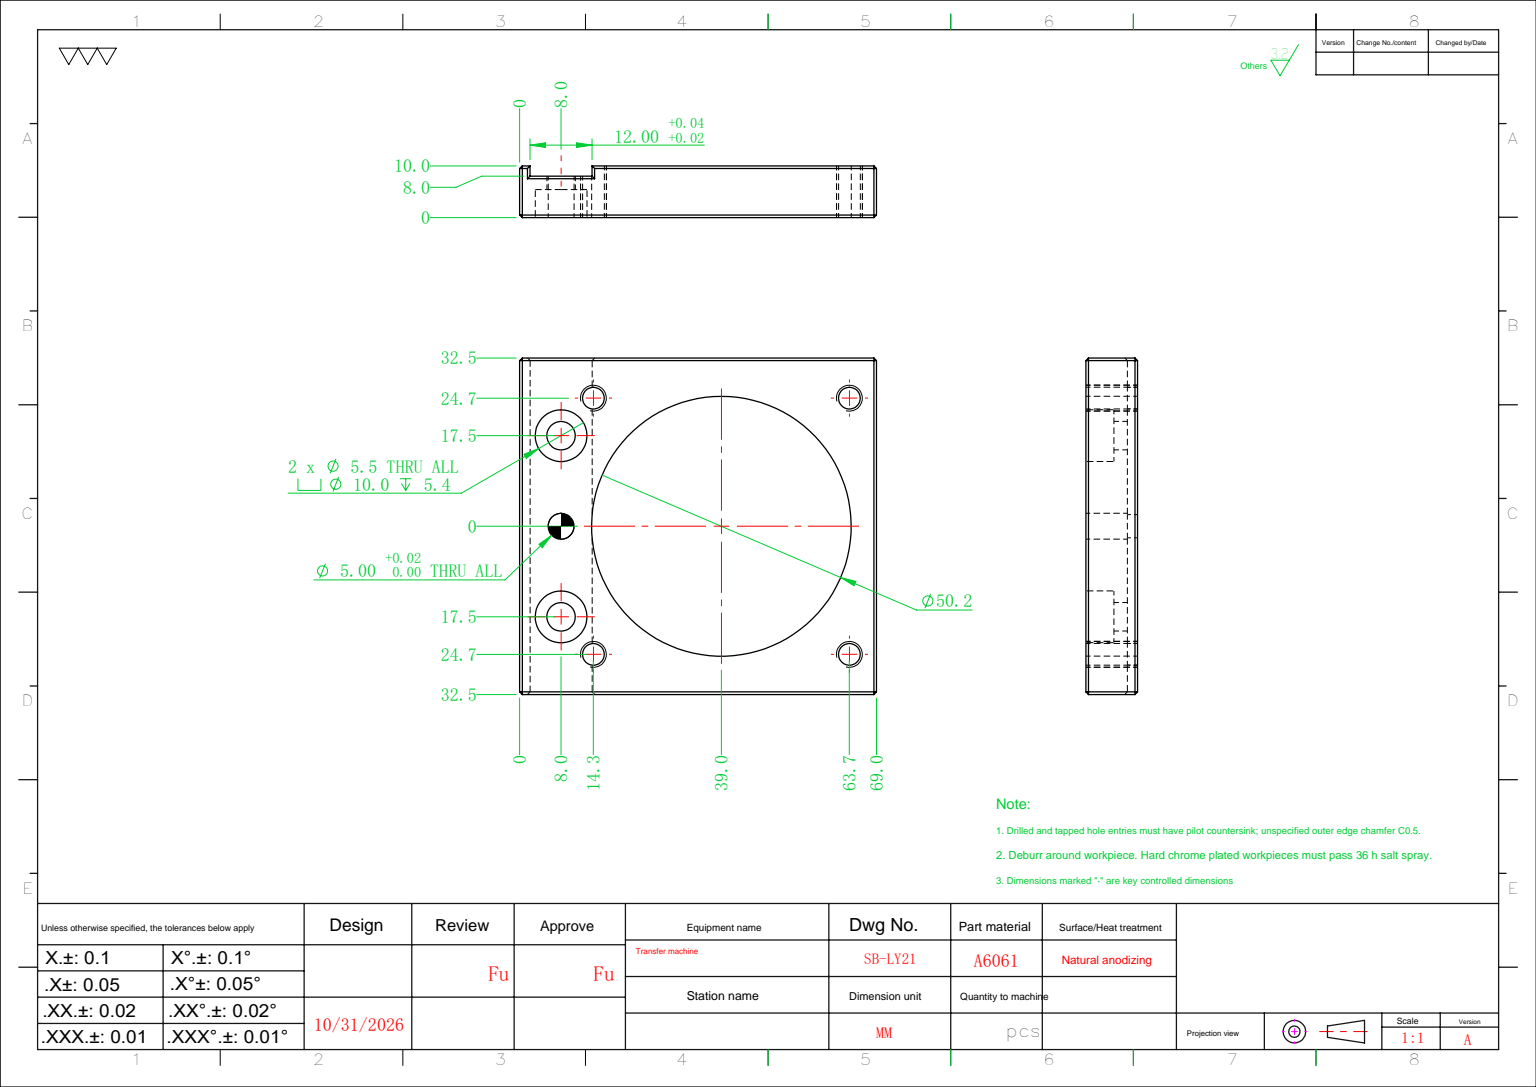
SolidWorks part; units mm, degrees
ref_plane "前视基准面" through (0, 0, 0) normal (0, 0, 1) x (1, 0, 0)
ref_plane "上视基准面" through (0, 0, 0) normal (0, 1, 0) x (1, 0, 0)
ref_plane "右视基准面" through (0, 0, 0) normal (1, 0, 0) x (0, 0, -1)
sketch "草图1" plane through (0, 0, 0) normal (0, 0, 1) x (1, 0, 0)
  line L1 (-32.5, -34.5) -> (32.5, -34.5)
  line L2 (-32.5, -34.5) -> (-32.5, 34.5)
  line L3 (-32.5, 34.5) -> (32.5, 34.5)
  line L4 (32.5, -34.5) -> (32.5, 34.5)
  line L5 (-32.5, -34.5) -> (32.5, 34.5) construction
  line L6 (-32.5, 34.5) -> (32.5, -34.5) construction
  point P0 (0, 0)
  dimension "D1" = 65
  dimension "D2" = 69
extrude "凸台-拉伸1" add sketch "草图1" along normal blind 10
sketch "草图2" plane through (-32.5, 0, 0) normal (-1, 0, 0) x (0, 0, 1)
  line L0 (0, 34.5) -> (0, -34.5) construction
  line L1 (0, 32.5) -> (2, 32.5)
  line L2 (0, 32.5) -> (0, 20.5)
  line L3 (0, 20.5) -> (2, 20.5)
  line L4 (2, 32.5) -> (2, 20.5)
  line L5 (10, 34.5) -> (0, 34.5) construction
  dimension "D1" = 12
  dimension "D2" = 2
  dimension "D3" = 2
extrude "切除-拉伸1" cut sketch "草图2" against normal through all
sketch "草图3" plane through (0, 0, 10) normal (0, 0, 1) x (1, 0, 0)
  line L0 (0, -34.5) -> (0, 34.5) construction
  line L1 (-32.5, -34.5) -> (32.5, -34.5) construction
  line L2 (32.5, 34.5) -> (-32.5, 34.5) construction
  circle A0 centre (0, -4.5) radius 25.1
  dimension "D1" = 50.2
  dimension "D2" = 39
extrude "切除-拉伸2" cut sketch "草图3" against normal through all
hole_wizard "M5 螺纹孔1" positions "草图4" profile "草图5" tap size "M5" standard "ISO" end condition through all
sketch "草图4" plane through (0, 0, 10) normal (0, 0, 1) x (1, 0, 0)
  line L0 (0, -4.5) -> (40.2684, -4.5) construction
  line L2 (0, -4.5) -> (0, 29.2508) construction
  point P0 (24.7487, 20.2487)
  point P3 (24.7487, -29.2487)
  point P6 (-24.7487, -29.2487)
  point P9 (-24.7487, 20.2487)
  dimension "D1" = 49.4975
  dimension "D2" = 49.4975
sketch "草图5" plane through (24.7487, 20.2487, 10) normal (1, 0, 0) x (0, -1, 0)
  line L0 (0, 0) -> (0, 10)
  line L1 (0, 10) -> (2.1, 10)
  line L2 (2.1, 10) -> (2.1, 0)
  line L5 (2.1, 0) -> (0, 0)
  line L11 (0, -6.35) -> (0, 107.95) construction
  dimension "通孔螺纹孔钻头直径" = 4.2
  dimension "通孔螺纹孔钻头深度" = 10
cosmetic thread "孔螺蚊线5" parameters "D2"=5
cosmetic thread "孔螺蚊线6" parameters "D2"=5
cosmetic thread "孔螺蚊线7" parameters "D2"=5
cosmetic thread "孔螺蚊线8" parameters "D2"=5
hole_wizard "M5 六角凹头螺钉的柱形沉头孔1" positions "草图6" profile "草图7" counterbore size "M5" standard "ISO" end condition through all
sketch "草图6" plane through (0, 0, 10) normal (0, 0, 1) x (1, 0, 0)
  line L0 (-32.5, 26.5) -> (32.5, 26.5) construction
  line L1 (-32.5, 20.5) -> (-32.5, 32.5) construction
  line L2 (32.5, 20.5) -> (32.5, 32.5) construction
  line L4 (0, 26.5) -> (0, 48.658) construction
  point P0 (17.5, 26.5)
  point P2 (-17.5, 26.5)
  dimension "D1" = 35
sketch "草图7" plane through (17.5, 26.5, 10) normal (1, 0, 0) x (0, -1, 0)
  line L0 (0, 0) -> (0, 10)
  line L1 (0, 10) -> (2.75, 10)
  line L3 (2.75, 10) -> (2.75, 5.4)
  line L4 (2.75, 5.4) -> (5, 5.4)
  line L5 (5, 5.4) -> (5, 0)
  line L7 (5, 0) -> (0, 0)
  line L11 (0, -6.35) -> (0, 107.95) construction
  dimension "通孔孔直径" = 5.5
  dimension "通孔孔深度" = 10
  dimension "柱形沉头孔直径" = 10
  dimension "柱形沉头孔深度" = 5.4
hole_wizard "大小mm 暗销孔1" positions "草图8" profile "草图9" hole size "Ø5.0" standard "ISO" end condition through all
sketch "草图8" plane through (0, 0, 10) normal (0, 0, 1) x (1, 0, 0)
  line L0 (17.5, 26.5) -> (-17.5, 26.5) construction
  point P0 (0, 26.5)
sketch "草图9" plane through (0, 26.5, 10) normal (1, 0, 0) x (0, -1, 0)
  line L0 (0, 0) -> (0, 10)
  line L1 (0, 10) -> (2.5, 10)
  line L2 (2.5, 10) -> (2.5, 0)
  line L5 (2.5, 0) -> (0, 0)
  line L11 (0, -6.35) -> (0, 107.95) construction
  dimension "通孔孔直径" = 5
  dimension "通孔孔深度" = 10
chamfer "倒角1" distance 0.5 angle 45 20 edges at (0, 34.5, 10) (0, 34.5, 0) (-32.5, 34.5, 5) (-32.5, 0, 10) (-32.5, 33.5, 0) (-32.5, 32.5, 1) (-32.5, 26.5, 2) (-32.5, 20.5, 1) (-32.5, -7, 0) (32.5, 20.5, 1) (32.5, -7, 0) (32.5, 26.5, 2) (32.5, 32.5, 1) (32.5, 33.5, 0) (32.5, 34.5, 5) (32.5, 0, 10) (-32.5, -34.5, 5) (0, -34.5, 10) (32.5, -34.5, 5) (0, -34.5, 0)
